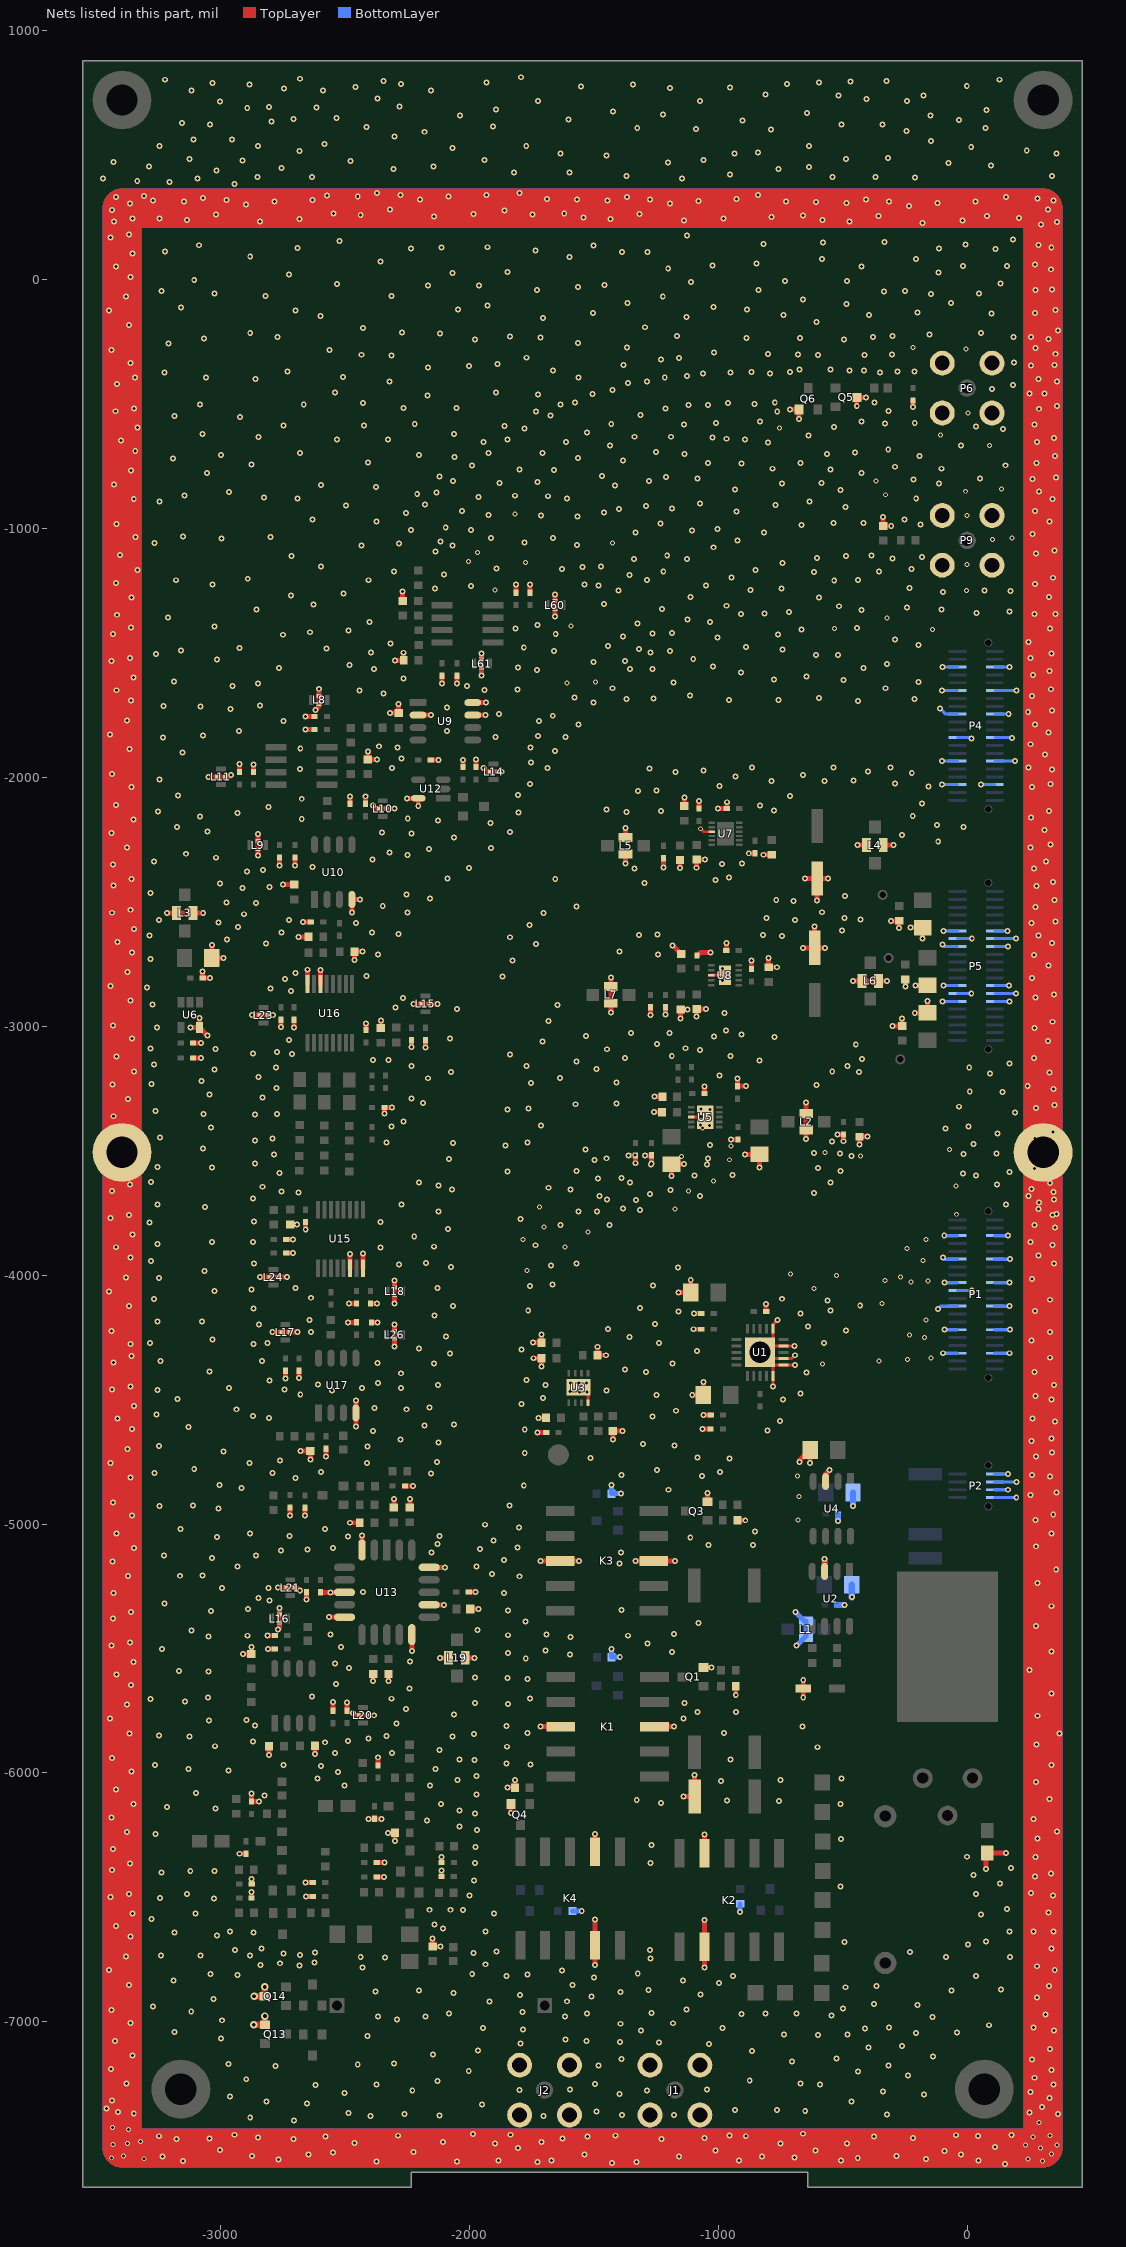
[diagram p0: the nets of this part, all layers, seen from the top]
# Altium PCB MISC109358.PcbDoc (part 3 of 7)
Units mil, origin at the board's own origin, x right, y up, seen from the top; angles counter-clockwise.
Board outline 4015.75 x 8543.31 mil, 4 copper layers (TopLayer, GND, POWER, BottomLayer), stack 33.234 mil thick; 299 components, 170 nets, 998 pads, 2318 vias.

## Via types
v1: diameter 24, hole 12, TopLayer to BottomLayer, 2184 vias
v2: diameter 20, hole 12, TopLayer to BottomLayer, 95 vias
v3: diameter 30, hole 15, TopLayer to BottomLayer, 37 vias
v4: diameter 40, hole 20, TopLayer to BottomLayer, 2 vias

## Nets (pads, with @x,y where several pads share a name; then routed paths per layer and width w, separated by ;. In a path a pad name is that pad's centre, name@x,y a point inside that pad or via, vN(x,y) a via of type N, cw(c..) or ccw(c..) an arc to the next point about the centre after c; other vN are vias at no path point) (continued)
GND: C3.2 C4.2 C5.2 C6.2 C7.2 C8.2 C9.2 C14.2 C15.2 C16.1 C17.1 C20.1 C21.1 C23.1 C24.2 C25.2 C26.2 C27.2 C28.2 C29.2 C30.2 C31.2 C32.2 C33.2 C34.2 C35.2 C36.2 C37.2 C38.1 C39.2 C40.1 C41.1 C42.2 C43.2 C45.1 C46.2 C47.2 C48.1 C49.1 C50.1 C51.2 C53.2 C54.2 C55.2 C57.1 C58.2 C59.1 C60.2 C61.1 C62.2 C63.2 C64.1 C65.1 C66.1 C67.2 C68.1 C69.2 C72.2 C73.2 C74.2 C75.1 C76.2 C77.1 C78.1 C79.1 C80.2 C81.1 C82.1 C83.2 C84.1 C85.1 C86.2 C89.1 C90.2 C91.2 C92.2 C93.1 C94.1 C96.2 C97.1 C99.1 C100.1 C101.2 C102.1 C103.1 C104.1 C105.1 C108.1 C110.1 C112.1 C113.2 C114.1 C115.2 C116.1 C117.1 C118.1 C120.1 C121.1 C122.1 C123.1 C124.2 C126.1 C127.1 C128.1 C129.1 C301.2 C302.1 C304.2 C305.1 C306.2 C307.1 C334.1 D10.1 J1.1 J1.2 J1.3 J1.4 J2.1 J2.2 J2.3 J2.4 K1.3 K1.8 K2.4 K2.7 K3.3 K3.8 K4.4 K4.7 L1.2 L1.4 L2.2 L2.4 L3.2 L3.4 L4.2 L4.4 L5.2 L5.4 L6.2 L6.4 L7.2 L7.4 L8.2 L9.2 L10.2 L11.2 L14.2 L15.2 L16.2 L17.2 L18.2 L19.2 L19.4 L20.2 L21.2 L23.2 L24.2 L26.2 L60.2 L61.2 P1.5 P1.6 P1.11 P1.12 P1.17 P1.18 P1.20 P1.23 P1.24 P1.29 P1.30 P1.35 P1.36 P2.1 P2.3 P2.5 P2.7 P4.5 P4.6 P4.11 P4.12 P4.17 P4.18 P4.23 P4.24 P4.29 P4.30 P4.35 P4.36 P5.11 P5.12 P5.13 P5.14 P5.15 P5.16 P5.25 P5.26 P5.27 P5.28 P5.29 P5.30 P6.1 P6.2 P6.3 P6.4 P9.1 P9.2 P9.3 P9.4 pad.3@305.27,-3506.52 pad.3@-3395.52,-3506.52 Q1.2 Q3.2 Q4.2 Q5.3 Q6.1 Q13.1 Q14.3 R2.2 R7.2 R9.2 R10.1 R15.2 R16.2 R17.1 R19.2 R20.2 R21.2 R22.2 R23.2 R24.2 R25.2 R34.2 R35.2 R36.2 R39.2 R40.1 R41.1 R42.1 R51.2 R60.1 R61.2 R63.1 R65.2 R66.1 R69.1 R71.1 R74.1 R75.1 R78.2 U1.5 U1.6 U1.7 U1.9 U1.11 U1.21 U2.3 U3.4 U3.9 U4.3 U5.8 U5.11 U6.5 U7.9 U8.8 U8.11 U9.2 U9.7 U9.8 U10.4 U12.5 U13.3 U13.6 U13.8 U13.13 U13.15 U13.18 U15.6 U15.8 U16.6 U16.8 U17.4 | length 61100.9
  TopLayer w10: v2(-1071.52,-2206.02) -1060.12,-2217.42 U7.9@-1026.16,-2217.42
  TopLayer w11: U5.8@-1107.68,-3364.63 U5.11@-1052.27,-3364.63
  TopLayer w12: U3.4@-1523.71,-4511.96 U3.9@-1523.71,-4478.52 ; U8.8@-1028.89,-2794.63 U8.11@-973.32,-2794.63 ; U1.21@-806.23,-4335.1 U1.7@-737.33,-4335.1 -706.1,-4335.1 v1(-692.52,-4321.52) ; U1.21@-806.23,-4283.92 U1.9@-737.33,-4283.92 v1(-694.52,-4283.92) ; v1(-780.64,-4446.64) U1.5@-780.64,-4404 -780.64,-4360.69 U1.6@-737.33,-4360.69 v1(-692.35,-4360.69) ; U1.21@-780.64,-4258.33 U1.11@-780.64,-4215.02 -780.64,-4198.64 v1(-762.52,-4180.52)
  TopLayer w20: v1(-3214.35,-2544.35) L3.2@-3176.98,-2544.35 L3.4@-3110.06,-2544.35 v1(-3069.35,-2544.35) ; v1(-3119.77,-3004.77) U6.5@-3084.61,-3004.77 ; C38.1@-3109.97,-3127.35 v1(-3078.35,-3127.35) ; C41.1@-3109.97,-3067.83 v1(-3078.66,-3067.83) ; v1(-3084.61,-2965.61) U6.5@-3084.61,-3004.77 ; v1(-3071.52,-2779.52) C40.1@-3071.52,-2806.52 v1(-3042.52,-2806.52) ; v1(-3052.86,-3036.52) U6.5@-3084.61,-3004.77 ; v1(-3047.54,-1997.5) L11.2@-3014.27,-1997.5 L11.2@-2982.77,-1997.5 -2965.5,-1997.5 v1(-2958.52,-1990.52) ; v1(-3034.52,-2672.52) C39.2@-3034.52,-2724.52 v1(-2987.52,-2724.52) ; C77.1@-2924.52,-1978.52 v1(-2924.52,-1945.52) ; v1(-2923,-6324.48) C92.2@-2897,-6324.48 ; v1(-2909.17,-5521.17) C110.1@-2875.52,-5521.17 v1(-2875.52,-5493.52) ; C82.1@-2875.04,-6502.04 v1(-2875.04,-6479.04) ; C83.2@-2874.52,-6446.52 v1(-2874.52,-6426.53) ; v1(-2874.52,-6081.52) C94.1@-2874.52,-6114.48 v1(-2845.52,-6114.48) ; v1(-2873.02,-2955.02) L23.2@-2843.27,-2955.02 L23.2@-2811.77,-2955.02 v1(-2788.52,-2955.02) ; C76.2@-2866.52,-1978.52 v1(-2866.52,-1946.94) ; v1(-2850.02,-2314.02) L9.2@-2850.02,-2287.27 L9.2@-2850.02,-2255.77 v1(-2850.02,-2228.02) ; v1(-2840.52,-4008.02) L24.2@-2803.27,-4008.02 L24.2@-2771.77,-4008.02 v1(-2732.02,-4008.02) ; v1(-2810.52,-5447.52) C104.1@-2781.52,-5447.52 ; v1(-2809.21,-5502) C105.1@-2782,-5502 ; v1(-2804.52,-5927.52) R71.1@-2804.52,-5892.52 ; v1(-2792.02,-4229.02) L17.2@-2755.27,-4229.02 L17.2@-2723.77,-4229.02 v1(-2690.02,-4229.02) ; v1(-2769.54,-5255.02) L21.2@-2735.27,-5255.02 L21.2@-2703.77,-5255.02 -2696.02,-5255.02 -2684.52,-5266.52 v1(-2680.52,-5266.52) ; v1(-2769.26,-5423.52) -2763.02,-5417.28 L16.2@-2763.02,-5395.27 L16.2@-2763.02,-5363.77 v1(-2763.02,-5337.02) ; v1(-2762.35,-2353.2) C69.2@-2762.35,-2321.09 ; v1(-2756.04,-3002.52) C124.2@-2756.04,-2973.04 ; v1(-2748.21,-2430.21) C72.2@-2704.52,-2430.21 ; v1(-2739.52,-4414.52) C99.1@-2739.52,-4384.04 ; C126.1@-2736,-3911.52 v1(-2708.52,-3911.52) ; C129.1@-2736,-3856.04 v1(-2708.56,-3856.04) ; v1(-2721.04,-4965.04) C116.1@-2721.04,-4933.52 ; R78.2@-2720.52,-3795.83 v1(-2691.83,-3795.83) ; v1(-2705.04,-3003.66) C123.1@-2705.04,-2973.04 ; v1(-2701.01,-2354.03) C68.1@-2701.01,-2321.09 ; v1(-2687.52,-2640.52) R40.1@-2646.52,-2640.52 ; v1(-2684.04,-4413.04) C102.1@-2684.04,-4384.04 ; v1(-2678.52,-4706.52) R75.1@-2638.52,-4706.52 v1(-2638.52,-4739.52) ; v1(-2668.52,-2581.52) C73.2@-2637.52,-2581.52 ; v1(-2661.04,-4965.04) C117.1@-2661.04,-4934.52 ; v1(-2659.04,-6440) C85.1@-2629,-6440 ; v1(-2658.47,-1754.08) C66.1@-2622,-1754.08 ; v1(-2658.04,-1808) C67.2@-2622,-1808 ; v1(-2657.52,-3815.52) C302.1@-2657.52,-3786.52 ; v1(-2656.04,-6496.48) C84.1@-2629,-6496.48 ; v1(-2653.52,-5303.52) C118.1@-2653.52,-5274.12 ; U16.8@-2650.14,-2830 v1(-2650.14,-2772.52) ; v1(-2620.77,-5924.27) R74.1@-2620.77,-5890.52 ; v1(-2617.52,-1728.52) -2617.52,-1727.52 -2603.5,-1713.5 L8.2@-2603.5,-1704.27 L8.2@-2603.5,-1672.77 v1(-2603.5,-1643.54) ; U16.6@-2598.96,-2830 v1(-2598.96,-2772.64) ; C120.1@-2598.67,-5274.12 C120.1@-2598.77,-5274.02 v1@-2559.02,-5274.02 ; v1(-2575.52,-4728.52) C115.2@-2575.52,-4697.21 ; v1(-2563.92,-5374.12) U13.8@-2501.46,-5374.12 ; v1(-2558.92,-5274.12) U13.6@-2501.46,-5274.12 ; C108.1@-2547.04,-5750 v1(-2547.04,-5714.04) ; C112.1@-2491.52,-5749.52 v1(-2491.52,-5716.52) ; v1(-2487,-4189) C121.1@-2453.52,-4189 ; v1(-2484.52,-4113.52) C128.1@-2453.52,-4113.52 ; v1(-2480.48,-4994.52) R66.1@-2440.52,-4994.52 ; C74.2@-2479.89,-2105.95 v1(-2479.89,-2076) ; U15.6@-2479.56,-3972.52 v1(-2479.56,-3914.56) ; v1(-2472,-2542.52) U10.4@-2472,-2490 v1(-2439.57,-2490) ; v1(-2467.52,-5758.4) -2457.9,-5768.02 L20.2@-2443.27,-5768.02 L20.2@-2411.77,-5768.02 v1(-2384.02,-5768.02) ; v1(-2461.52,-2732.52) R41.1@-2461.52,-2699.52 v1(-2428.52,-2699.52) ; v1(-2456,-4607) U17.4@-2456,-4553 v1(-2456,-4504.04) ; U13.3@-2431.46,-5104.12 v1(-2431.46,-5045.58) ; U15.8@-2428.38,-3972.52 v1(-2428.38,-3912.66) ; C75.1@-2416.55,-2105.95 v1(-2416.55,-2075.49) ; C301.2@-2414.52,-3014.52 v1(-2414.52,-2988.52) ; v1(-2407.52,-1895.52) R36.2@-2407.52,-1927.21 v1(-2370.83,-1927.21) ; v1(-2406,-6184) C91.2@-2380.52,-6184 v1(-2354.04,-6184) ; C127.1@-2396.52,-4113.52 v1(-2371.52,-4113.52) ; C122.1@-2394.08,-4189.52 v1(-2368.52,-4189.52) ; v1(-2387.52,-2113.52) -2376.02,-2125.02 L10.2@-2363.83,-2125.02 L10.2@-2332.33,-2125.02 v1(-2301.52,-2125.02) ; v1(-2387,-5631.04) R69.1@-2387,-5601.54 ; C79.1@-2372.52,-6417.52 v1(-2343,-6417.52) ; C78.1@-2372.52,-6360.52 v1(-2341.52,-6360.52) ; C93.1@-2368.04,-5969.48 v1(-2368.04,-5936.77) ; R63.1@-2355.52,-3006.52 v1(-2355.52,-2976.52) ; v1(-2341.52,-3350.52) C103.1@-2341.52,-3325.52 v1(-2310.52,-3325.52) ; v1(-2327,-6241) R51.2@-2298.83,-6241 v1(-2298.83,-6272.67) ; v1(-2325,-5631.04) R65.2@-2325,-5601.54 ; v1(-2319.21,-1741.21) R39.2@-2284.52,-1741.21 v1(-2284.52,-1704.52) ; R60.1@-2302.99,-4933.52 v1(-2302.99,-4898.99) ; v1(-2301.02,-4286.02) L26.2@-2301.02,-4254.75 L26.2@-2301.02,-4223.25 v1(-2301.02,-4197.02) ; v1(-2300.02,-4113.52) L18.2@-2300.02,-4080.27 L18.2@-2300.02,-4048.77 v1(-2300.02,-4022.02) ; v1(-2299.02,-1529.52) R34.2@-2263.83,-1529.52 v1(-2263.83,-1498.83) ; R35.2@-2268.52,-1290.52 v1(-2268.52,-1252.52) ; C97.1@-2258.52,-4847.52 v1(-2227.08,-4847.52) ; v1(-2249.83,-2083.64) U12.5@-2205.42,-2083.64 v1(-2205.42,-2114.42) ; R61.2@-2238.99,-4933.21 v1(-2238.99,-4899.99) ; v1(-2232.02,-3083.65) C101.2@-2232.02,-3055.52 ; v1(-2231.46,-5510.52) U13.13@-2231.46,-5444.12 ; v1(-2225.02,-2910.02) L15.2@-2192.27,-2910.02 L15.2@-2160.77,-2910.02 v1(-2127.52,-2910.02) ; U9.2@-2206.52,-1749.52 v1(-2153.52,-1749.52) ; v1(-2176.52,-3084.52) C100.1@-2176.52,-3055.52 ; U13.15@-2161.46,-5324.12 v1(-2102.51,-5324.12) ; U13.18@-2161.46,-5174.12 v1(-2098.52,-5174.12) ; C86.2@-2155.52,-1930.52 v1(-2124.52,-1930.52) ; v1(-2147.52,-6665.52) R42.1@-2147.52,-6696.52 v1(-2116.52,-6696.52) ; v1(-2118.35,-5537.35) L19.2@-2083.5,-5537.35 ; C80.2@-2112.52,-6415.52 v1(-2112.52,-6391) ; C81.1@-2112.04,-6359 v1(-2112.04,-6337.04) ; v1(-2109.23,-1622.81) C304.2@-2109.23,-1590.99 ; v1(-2050.52,-1622.04) C305.1@-2050.52,-1591.04 ; C89.1@-2025.04,-1958.46 v1(-2025.04,-1929.04) ; L19.4@-2016.58,-5537.35 v1(-1978.52,-5537.35) ; C114.1@-2002.52,-5273.52 v1(-1975.52,-5273.52) ; C113.2@-1996.4,-5340.52 v1(-1963.52,-5340.52) ; U9.7@-1986.52,-1749.52 v1(-1935.52,-1749.52) ; U9.8@-1986.52,-1699.52 v1(-1932.52,-1699.52) ; C90.2@-1973.04,-1958.46 v1(-1973.04,-1928.04) ; v1(-1951.02,-1589.54) L61.2@-1951.02,-1558.27 L61.2@-1951.02,-1526.77 v1(-1951.02,-1502.5) ; v1(-1943.52,-1961.52) -1928.02,-1977.02 L14.2@-1918.27,-1977.02 L14.2@-1886.77,-1977.02 v1(-1870.02,-1977.02) ; v1(-1847.31,-6058.52) R17.1@-1817.04,-6058.52 v1(-1817.04,-6029.04) ; v1(-1832.52,-6160.52) Q4.2@-1832.52,-6124.52 ; C306.2@-1813.52,-1257.48 v1(-1813.52,-1225.52) ; C307.1@-1757.31,-1257.48 v1(-1757.31,-1224.93) ; v1(-1744.48,-4270.52) C23.1@-1709.79,-4270.52 v1(-1709.79,-4237.79) ; v1(-1741.52,-4333.52) C24.2@-1709.79,-4333.52 v1(-1709.79,-4366.52) ; v1(-1726.52,-4632.48) C25.2@-1691.48,-4632.48 ; v1(-1722.52,-4572.96) C26.2@-1691.79,-4572.96 ; v1(-1714.52,-5148.14) K3.3@-1635.12,-5148.14 v1(-1560.14,-5148.14) ; v1(-1713.52,-5814.14) K1.3@-1632.12,-5814.14 ; v1(-1656.02,-1354.02) L60.2@-1656.02,-1323.23 L60.2@-1656.02,-1291.73 v1(-1656.02,-1264.02) ; v1(-1495.46,-6771.46) K4.4@-1495.46,-6692.12 v1(-1495.46,-6589.58) ; K4.7@-1495.46,-6316.12 v1(-1495.46,-6244.46) ; v1(-1485.21,-4287.36) C27.2@-1485.21,-4321.52 v1(-1451.52,-4321.52) ; v1(-1431.83,-2944.21) L7.4@-1431.83,-2906.98 L7.2@-1431.83,-2840.06 v1(-1431.83,-2803.52) ; v1(-1423.48,-4660.52) R15.2@-1423.48,-4625.27 v1(-1384.77,-4625.27) ; v1(-1372.35,-2345.35) L5.4@-1372.35,-2307.98 ; L5.2@-1372.35,-2241.06 v1(-1372.35,-2202.23) ; v1(-1360.52,-3518.52) C36.2@-1333.02,-3518.52 v1(-1333.02,-3550.02) ; v1(-1332.9,-5148.14) K3.8@-1259.12,-5148.14 v1(-1173.14,-5148.14) ; v1(-1294.83,-3518.21) C37.2@-1268.4,-3518.21 v1(-1268.4,-3551.52) ; v1(-1271.75,-2953.75) C58.2@-1271.75,-2923.52 ; v1(-1258.73,-3344.73) R20.2@-1225.69,-3344.73 ; v1(-1256.81,-3282.73) C31.2@-1224.69,-3282.73 ; K1.8@-1256.12,-5814.14 v1(-1176.9,-5814.14) ; v1(-1219.27,-2361.26) C47.2@-1219.27,-2324.52 ; v1(-1212.75,-2951.59) C63.2@-1212.75,-2923.52 ; v1(-1187.26,-3600.78) C30.2@-1187.26,-3553.69 v1(-1137.69,-3553.69) ; v1(-1183.52,-2674.52) C65.1@-1149.52,-2708.52 ; v1(-1160.52,-4069.52) C3.2@-1110.52,-4069.52 v1(-1110.52,-4018.52) ; v1(-1153.75,-2364.29) C334.1@-1153.75,-2332.28 ; v1(-1151.23,-2968.81) C61.1@-1151.23,-2932 v1(-1123,-2932) ; v1(-1139.52,-6094.52) R2.2@-1094.96,-6094.52 v1(-1094.96,-6007.96) ; C53.2@-1136.52,-2114.52 v1(-1136.52,-2080.58) ; v1(-1104.52,-4481.52) C7.2@-1059.52,-4481.52 v1(-1059.52,-4428.52) ; v1(-1099.04,-4217) C4.2@-1068,-4217 ; v1(-1097.52,-4153.52) C5.2@-1068.52,-4153.52 ; v1(-1087.23,-2961.23) C64.1@-1087.23,-2931 v1(-1049,-2931) ; v1(-1086.75,-2362.75) C48.1@-1086.75,-2330.28 v1(-1052.52,-2330.28) ; R25.2@-1084.58,-2715.83 -1083.83,-2715.83 -1071.52,-2703.52 v1(-1031.52,-2703.52) ; R23.2@-1077,-2124.59 v1(-1077,-2094.06) ; v1(-1062.52,-4618.52) C9.2@-1031,-4618.52 ; v1(-1059.52,-4561.52) C8.2@-1030.52,-4561.52 ; Q1.2@-1058.52,-5576.52 v1(-1027.52,-5576.52) ; v1(-1055.14,-6781.52) K2.7@-1055.14,-6698.4 v1(-1055.14,-6590.52) ; K2.4@-1055.14,-6322.4 v1(-1055.14,-6247.9) ; R19.2@-1054.9,-3270.21 v1(-1054.9,-3241.1) ; Q3.2@-1044,-4910 v1(-1044,-4874.04) ; v1(-1000.52,-2125.52) R22.2@-965.52,-2125.52 v1(-965.52,-2099.52) ; R24.2@-967.75,-2695.52 v1(-967.75,-2665.29) ; v1(-948.52,-3454.52) C32.2@-920.52,-3454.52 ; v1(-929.69,-5687.35) R7.2@-929.69,-5651.04 ; v1(-923.52,-3209.52) R21.2@-923.52,-3240.52 v1(-888.52,-3240.52) ; R16.2@-922.69,-4984.52 v1(-891.52,-4984.52) ; v1(-892.48,-3514.52) C33.2@-834.52,-3514.52 v1(-834.52,-3567.52) ; v1(-877.52,-2304.52) C46.2@-852.52,-2304.52 ; C60.2@-865.75,-2770 v1(-865.75,-2736.29) ; v1(-818.02,-2310.52) C45.1@-785.52,-2310.52 ; C6.2@-807.41,-4146.52 v1(-807.41,-4115.41) ; v1(-797.52,-2726.02) C59.1@-797.52,-2762.52 v1(-763.52,-2762.52) ; v1(-711.52,-520.89) Q6.1@-675.52,-520.89 v1(-675.52,-558.89) ; v1(-673.52,-4749.52) -673.52,-4744.52 R9.2@-630.52,-4701.52 v1(-630.52,-4754.52) ; v1(-658.76,-2684.28) C62.2@-612.52,-2684.28 ; v1(-658.53,-5697.51) D10.1@-658.53,-5661.39 v1(-658.53,-5626.51) ; v1(-652.1,-2405.52) C49.1@-602.52,-2405.52 ; v1(-646.55,-3452.55) L2.2@-646.55,-3416.55 L2.4@-646.55,-3349.63 v1(-646.55,-3306.55) ; v1(-612.52,-2598.52) C62.2@-612.52,-2684.28 ; v1(-602.52,-2493.52) C49.1@-602.52,-2405.52 ; v1(-570.76,-2684.28) C62.2@-612.52,-2684.28 ; U4.3@-568.51,-4828.65 -568.51,-4798.51 v1(-552.52,-4782.52) ; v1(-558.2,-2405.52) C49.1@-602.52,-2405.52 ; v1(-519.96,-3434.09) C34.2@-497.38,-3434.09 v1(-497.38,-3461.66) ; v1(-457.69,-2817.35) L6.2@-422.98,-2817.35 L6.4@-356.06,-2817.35 v1(-321.35,-2817.35) ; v1(-443.52,-506.89) Q5.3@-443.52,-472.87 v1(-406.54,-472.87) ; v1(-439.69,-2271.69) L4.4@-403.98,-2271.69 ; v1(-432.52,-3474.52) C35.2@-432.52,-3443.4 v1(-400.8,-3443.4) ; v1(-337.61,-953.18) C96.2@-337.61,-988.87 v1(-304.92,-988.87) ; L4.2@-337.06,-2271.69 v1(-296.64,-2271.69) ; v1(-305.21,-2575.83) C43.2@-273.52,-2575.83 v1(-273.52,-2604.52) ; v1(-300.21,-2998.21) C54.2@-261.52,-2998.21 v1(-261.52,-2968.52) ; v1(-248.52,-2840.06) C50.1@-248.52,-2811.52 ; v1(-227.52,-2603.52) C42.2@-178.49,-2603.52 v1(-178.49,-2646.52) ; v1(-217,-511.89) C57.1@-217,-485.37 ; v1(-210.52,-2945.52) C55.2@-159.52,-2945.52 v1(-159.52,-2897.52) ; v1(-208.02,-2835.52) -159.94,-2835.52 C51.2@-158.52,-2834.09 ; v1(75.48,-6385.52) 75.48,-6326.52 R10.1@80.48,-6321.52 v1(156.48,-6321.52)
  TopLayer w25: v3(-2866.52,-7011.52) Q13.1@-2821.58,-7011.52 v3(-2821.58,-6976.58) ; v3(-2865.02,-6897.02) Q14.3@-2822.58,-6897.02 v3(-2822.58,-6859.52) ; U2.3@-572.51,-5190.24 v1(-572.51,-5140.53)
  TopLayer w157.48: -3395.52,-7506.52 305.27,-7506.52 305.27,287.48 -3395.52,287.48 pad.3@-3395.52,-3506.52 -3395.52,-7506.52
  BottomLayer w12: v1(-108.52,-1722.61) -85.64,-1745.49 P4.18@-38.57,-1745.49 ; v1(-101.57,-1934.46) P4.30@-38.57,-1934.46 ; v1(-101.09,-2028.95) P4.36@-38.57,-2028.95 ; v1(-100.61,-1651) P4.12@-38.57,-1651 ; v1(-99.52,-2671.52) -91.94,-2679.1 P5.16@-38.57,-2679.1 ; v1(-98.51,-1556.51) P4.6@-38.57,-1556.51 ; v1(-98.26,-2899.57) P5.30@-38.57,-2899.57 ; v1(-95.46,-2836.58) P5.26@-38.57,-2836.58 ; v1(-94.93,-2616.11) P5.12@-38.57,-2616.11 ; P5.28@-38.57,-2868.08 v1(16.54,-2868.08) ; P5.14@-38.57,-2647.61 v1(18.57,-2647.61) ; P4.24@-38.57,-1839.98 14.94,-1839.98 v1(17.48,-1842.52) ; v1(55.05,-2028.95) P4.35@111.04,-2028.95 ; P5.29@111.04,-2899.57 v1(169.34,-2899.57) ; P5.27@111.04,-2868.08 v1(196.5,-2868.08) ; P5.25@111.04,-2836.58 v1(168.29,-2836.58) ; P5.15@111.04,-2679.1 v1(165.08,-2679.1) ; P5.13@111.04,-2647.61 v1(196.5,-2647.61) ; P5.11@111.04,-2616.11 v1(162.89,-2616.11) ; P4.29@111.04,-1934.46 v1(191.54,-1934.46) ; P4.23@111.04,-1839.98 185.02,-1839.98 184.48,-1840.52 v1(179.48,-1840.52) ; P4.17@111.04,-1745.49 v1(167.14,-1745.49) ; P4.11@111.04,-1651 v1(197.58,-1651) ; P4.5@111.04,-1556.51 v1(170.88,-1556.51)
  BottomLayer w13: v1(-117.52,-4136.52) -105.46,-4124.46 P1.24@-38.57,-4124.46 ; v1(-97.52,-3928.52) -90.56,-3935.48 P1.12@-38.57,-3935.48 ; v1(-96.61,-4313.43) P1.36@-38.57,-4313.43 ; v1(-91.99,-3840.99) P1.6@-38.57,-3840.99 ; v1(-91.42,-4218.94) P1.30@-38.57,-4218.94 ; v1(-90.56,-4029.97) P1.18@-38.57,-4029.97 ; P1.20@-38.57,-4061.46 v1(18.54,-4061.46) ; P2.1@111.04,-4893.41 v1(197.37,-4893.41) ; P2.3@111.04,-4861.91 v1(164.09,-4861.91) ; P2.5@111.04,-4830.42 v1(197.58,-4830.42) ; P2.7@111.04,-4798.92 v1(165.08,-4798.92) ; P1.35@111.04,-4313.43 v1(169.39,-4313.43) ; P1.29@111.04,-4218.94 v1(172.06,-4218.94) ; P1.23@111.04,-4124.46 v1(170.89,-4124.46) ; P1.17@111.04,-4029.97 v1(170.89,-4029.97) ; P1.11@111.04,-3935.48 v1(171.44,-3935.48) ; P1.5@111.04,-3840.99 v1(165.01,-3840.99)
  BottomLayer w20: v1@-2682.48,-5268.48 v1(-2680.52,-5266.52) ; v1@-2618.52,-1728.52 v1(-2617.52,-1728.52) ; C21.1@-1585.52,-6554.52 v1(-1548.52,-6554.52) ; v1(-1429.52,-4842.52) C20.1@-1429.52,-4877.52 v1(-1391.52,-4877.52) ; v1(-1428.52,-5501.69) C16.1@-1428.52,-5534.52 v1(-1395.77,-5534.52) ; v1(-1136.52,-2080.58) v1@-1134.77,-2078.83 ; v1(-912.52,-6559) C17.1@-912.52,-6525.52 ; v1(-689.52,-5353.52) -653.98,-5389.06 L1.2@-647.69,-5389.06 -647.69,-5450.69 v1(-685.52,-5488.52)
  BottomLayer w25: C28.2@-522.51,-5325.11 v1(-492.52,-5325.11) ; v1(-518.52,-4987.52) C14.2@-518.52,-4964.52 ; v1(-463.52,-5293.52) C29.2@-463.52,-5243.52 ; v1(-458.52,-4926.52) C15.2@-458.52,-4872.52
  BottomLayer w157.48: -3395.52,-7506.52 pad.3@-3395.52,-3506.52 -3395.52,287.48 305.27,287.48 305.27,-7506.52 -3395.52,-7506.52